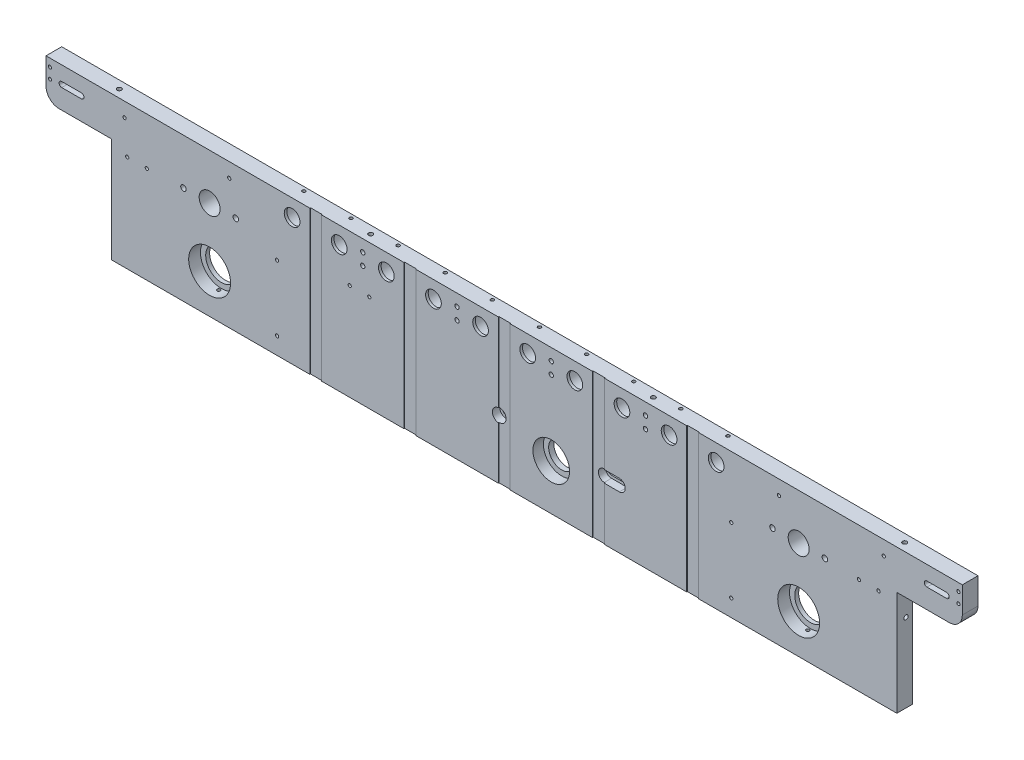
from build123d import *

# Parameters (mm, degrees)
EXTRUDE_1_DEPTH           = 12
FILLET_1_R                = 10
SKETCH_4_R                = 16
CUT_EXTRUDE_3_DEPTH       = 9
SKETCH_6_R                = 7.5
CUT_EXTRUDE_4_DEPTH       = 10
SKETCH_7_R                = 5.5
CUT_EXTRUDE_5_DEPTH       = 368.074924232
CUT_EXTRUDE_6_DEPTH       = 368.074924232
SKETCH_12_R               = 14
CUT_EXTRUDE_7_DEPTH       = 8
SKETCH_13_R               = 10
CUT_EXTRUDE_8_DEPTH       = 367.965938474
HOLE_WIZARD_M3_2_REACH    = 369.075
HOLE_WIZARD_M3_2_BORE_R   = 1.25
HOLE_WIZARD_M3_4_D        = 2.5
HOLE_WIZARD_2_D           = 5.5
HOLE_WIZARD_2_CBORE_D     = 10
HOLE_WIZARD_2_CBORE_DEPTH = 5.7
CUT_EXTRUDE_9_DEPTH       = 368.074924262
CUT_EXTRUDE_10_DEPTH      = 6
HOLE_WIZARD_M4_2_D        = 3.3
HOLE_WIZARD_M4_2_DEPTH    = 10
HOLE_WIZARD_M4_2_TIP      = 0.991420021
HOLE_WIZARD_M4_3_D        = 3.3
HOLE_WIZARD_M4_3_DEPTH    = 10.1
HOLE_WIZARD_M4_3_TIP      = 0.991420021
HOLE_WIZARD_M4_4_D        = 3.3
HOLE_WIZARD_M4_4_DEPTH    = 12.1
HOLE_WIZARD_M4_4_TIP      = 0.991420021
HOLE_WIZARD_M3_5_D        = 2.5
SKETCH_38_R               = 12
CUT_EXTRUDE_11_DEPTH      = 367.989100688
SKETCH_39_W               = 9
SKETCH_39_H               = 0.5
CUT_EXTRUDE_12_DEPTH      = 368.074924265
HOLE_WIZARD_M4_5_D        = 3.3
HOLE_WIZARD_M4_5_DEPTH    = 12
HOLE_WIZARD_M4_5_TIP      = 0.991420021
HOLE_WIZARD_M3_6_REACH    = 369.075
HOLE_WIZARD_M3_6_BORE_R   = 1.25
SKETCH_44_R               = 8
CUT_EXTRUDE_13_DEPTH      = 368.074924265
HOLE_WIZARD_M5_1_D        = 4.2
HOLE_WIZARD_3_D           = 2.4
HOLE_WIZARD_3_CBORE_D     = 4.3
HOLE_WIZARD_3_CBORE_DEPTH = 2.3
HOLE_WIZARD_4_D           = 2.4
HOLE_WIZARD_4_CBORE_D     = 4.3
HOLE_WIZARD_4_CBORE_DEPTH = 2.3
SKETCH_51_R               = 1.6
CUT_EXTRUDE_14_DEPTH      = 368.074924265
HOLE_WIZARD_M4_6_D        = 3.3
HOLE_WIZARD_5_D           = 12
HOLE_WIZARD_5_CBORE_D     = 16
HOLE_WIZARD_5_CBORE_DEPTH = 10
HOLE_WIZARD_M3_7_D        = 2.5


with BuildPart() as part:
    # 草图1 → 凸台-拉伸1 (new body)
    with BuildSketch(Plane.XY):
        Polygon((-350, -30), (-300, -30), (-300, -110), (300, -110), (300, -30), (350, -30), (350, 0), (-350, 0), align=None)
    extrude(amount=EXTRUDE_1_DEPTH)

    # 圆角1
    fillet_1_edges = [part.edges().sort_by_distance(p)[0] for p in [
        (350, -30, 6),
        (-350, -30, 6),
    ]]
    fillet(fillet_1_edges, radius=FILLET_1_R)

    # 草图4 → 切除-拉伸3 (cut)
    with BuildSketch(Plane.XY.offset(12)):
        with Locations((-225, -80)):
            Circle(SKETCH_4_R)
        with Locations(Location((225, -80, 0), (0, 0, 180))):
            Circle(SKETCH_4_R)
    extrude(amount=-CUT_EXTRUDE_3_DEPTH, mode=Mode.SUBTRACT)

    # 草图6 → 切除-拉伸4 (cut)
    with BuildSketch(Plane(origin=(0, 0, 0), x_dir=(-1, 0, 0), z_dir=(0, 0, -1))):
        with Locations((-162, -13)):
            Circle(SKETCH_6_R)
        with Locations((-126, -13)):
            Circle(SKETCH_6_R)
        with Locations((-90, -13)):
            Circle(SKETCH_6_R)
        with Locations((-54, -13)):
            Circle(SKETCH_6_R)
        with Locations((-18, -13)):
            Circle(SKETCH_6_R)
        with Locations((18, -13)):
            Circle(SKETCH_6_R)
        with Locations((54, -13)):
            Circle(SKETCH_6_R)
        with Locations((90, -13)):
            Circle(SKETCH_6_R)
        with Locations((126, -13)):
            Circle(SKETCH_6_R)
        with Locations((162, -13)):
            Circle(SKETCH_6_R)
    extrude(amount=-CUT_EXTRUDE_4_DEPTH, mode=Mode.SUBTRACT)

    # 草图7 → 切除-拉伸5 (cut, through all)
    with BuildSketch(Plane(origin=(0, 0, 0), x_dir=(-1, 0, 0), z_dir=(0, 0, -1))):
        with Locations((-162, -13)):
            Circle(SKETCH_7_R)
        with Locations((-126, -13)):
            Circle(SKETCH_7_R)
        with Locations((-90, -13)):
            Circle(SKETCH_7_R)
        with Locations((-54, -13)):
            Circle(SKETCH_7_R)
        with Locations((-18, -13)):
            Circle(SKETCH_7_R)
        with Locations((18, -13)):
            Circle(SKETCH_7_R)
        with Locations((54, -13)):
            Circle(SKETCH_7_R)
        with Locations((90, -13)):
            Circle(SKETCH_7_R)
        with Locations((126, -13)):
            Circle(SKETCH_7_R)
        with Locations((162, -13)):
            Circle(SKETCH_7_R)
    extrude(amount=-CUT_EXTRUDE_5_DEPTH, mode=Mode.SUBTRACT)

    # 草图8 → 切除-拉伸6 (cut, through all)
    with BuildSketch(Plane(origin=(0, 0, 0), x_dir=(-1, 0, 0), z_dir=(0, 0, -1))):
        with BuildLine():
            Line((-338, -11), (-323, -11))
            ThreePointArc((-323, -11), (-321, -13), (-323, -15))
            Line((-323, -15), (-338, -15))
            ThreePointArc((-338, -15), (-340, -13), (-338, -11))
        make_face()
        with BuildLine():
            Line((338, -11), (323, -11))
            ThreePointArc((323, -11), (321, -13), (323, -15))
            Line((323, -15), (338, -15))
            ThreePointArc((338, -15), (340, -13), (338, -11))
        make_face()
    extrude(amount=-CUT_EXTRUDE_6_DEPTH, mode=Mode.SUBTRACT)

    # 草图12 → 切除-拉伸7 (cut)
    with BuildSketch(Plane.XY.offset(12)):
        with Locations((36, -75)):
            Circle(SKETCH_12_R)
    extrude(amount=-CUT_EXTRUDE_7_DEPTH, mode=Mode.SUBTRACT)

    # 草图13 → 切除-拉伸8 (cut, through all)
    with BuildSketch(Plane.XY.offset(4)):
        with Locations((36, -75)):
            Circle(SKETCH_13_R)
    extrude(amount=-CUT_EXTRUDE_8_DEPTH, mode=Mode.SUBTRACT)

    # M3 螺纹孔2 bore → M3 螺纹孔2 (cut, up to next)
    with BuildSketch(Plane(origin=(0, -110, 0), x_dir=(-1, 0, 0), z_dir=(0, -1, 0)), mode=Mode.PRIVATE) as hole_wizard_m3_2_sk1:
        with Locations((225, -5)):
            Circle(HOLE_WIZARD_M3_2_BORE_R)
    hole_wizard_m3_2_tool1 = extrude(hole_wizard_m3_2_sk1.sketch, amount=-HOLE_WIZARD_M3_2_REACH, mode=Mode.PRIVATE) & part.part
    # M3 螺纹孔2 bore → M3 螺纹孔2 (cut, up to next)
    with BuildSketch(Plane(origin=(0, -110, 0), x_dir=(-1, 0, 0), z_dir=(0, -1, 0)), mode=Mode.PRIVATE) as hole_wizard_m3_2_sk2:
        with Locations((-225, -5)):
            Circle(HOLE_WIZARD_M3_2_BORE_R)
    hole_wizard_m3_2_tool2 = extrude(hole_wizard_m3_2_sk2.sketch, amount=-HOLE_WIZARD_M3_2_REACH, mode=Mode.PRIVATE) & part.part
    add(hole_wizard_m3_2_tool1.solids().sort_by_distance((-225, -110, 5))[0], mode=Mode.SUBTRACT)
    add(hole_wizard_m3_2_tool2.solids().sort_by_distance((225, -110, 5))[0], mode=Mode.SUBTRACT)

    # M3 螺纹孔4 (through all)
    with Locations(Plane.XY.offset(12)):
        with Locations((290, -11), (210, -11), (-210, -11), (-290, -11)):
            Hole(HOLE_WIZARD_M3_4_D / 2)

    # 打孔尺寸根据内六角圆柱头螺钉的类型2 (through all)
    with Locations(Plane.XY.offset(12)):
        with Locations((-4, -65)):
            CounterBoreHole(HOLE_WIZARD_2_D / 2, HOLE_WIZARD_2_CBORE_D / 2, HOLE_WIZARD_2_CBORE_DEPTH)

    # 草图28 → 切除-拉伸9 (cut, through all)
    with BuildSketch(Plane.XY.offset(12)):
        with BuildLine():
            Line((76, -62.5), (88, -62.5))
            ThreePointArc((88, -62.5), (90.5, -65), (88, -67.5))
            Line((88, -67.5), (76, -67.5))
            ThreePointArc((76, -67.5), (73.5, -65), (76, -62.5))
        make_face()
    extrude(amount=-CUT_EXTRUDE_9_DEPTH, mode=Mode.SUBTRACT)

    # 草图29 → 切除-拉伸10 (cut)
    with BuildSketch(Plane.XY.offset(12)):
        with BuildLine():
            Line((76, -60.5), (88, -60.5))
            ThreePointArc((88, -60.5), (92.5, -65), (88, -69.5))
            Line((88, -69.5), (76, -69.5))
            ThreePointArc((76, -69.5), (71.5, -65), (76, -60.5))
        make_face()
    extrude(amount=-CUT_EXTRUDE_10_DEPTH, mode=Mode.SUBTRACT)

    # M4 螺纹孔2
    with Locations(Plane(origin=(300, 0, 0), x_dir=(0, 0, -1), z_dir=(1, 0, 0))):
        with Locations((-5, -50)):
            Hole(HOLE_WIZARD_M4_2_D / 2, depth=HOLE_WIZARD_M4_2_DEPTH)
            with Locations((0, 0, -(HOLE_WIZARD_M4_2_DEPTH + HOLE_WIZARD_M4_2_TIP / 2))):  # 118° drill point
                Cone(0, HOLE_WIZARD_M4_2_D / 2, HOLE_WIZARD_M4_2_TIP, mode=Mode.SUBTRACT)

    # M4 螺纹孔3
    with Locations(Plane.ZY.offset(300)):
        with Locations((5, -50)):
            Hole(HOLE_WIZARD_M4_3_D / 2, depth=HOLE_WIZARD_M4_3_DEPTH)
            with Locations((0, 0, -(HOLE_WIZARD_M4_3_DEPTH + HOLE_WIZARD_M4_3_TIP / 2))):  # 118° drill point
                Cone(0, HOLE_WIZARD_M4_3_D / 2, HOLE_WIZARD_M4_3_TIP, mode=Mode.SUBTRACT)

    # M4 螺纹孔4
    with Locations(Plane(origin=(0, -110, 0), x_dir=(-1, 0, 0), z_dir=(0, -1, 0))):
        with Locations((262, -5), (82, -5), (-82, -5), (-262, -5)):
            Hole(HOLE_WIZARD_M4_4_D / 2, depth=HOLE_WIZARD_M4_4_DEPTH)
            with Locations((0, 0, -(HOLE_WIZARD_M4_4_DEPTH + HOLE_WIZARD_M4_4_TIP / 2))):  # 118° drill point
                Cone(0, HOLE_WIZARD_M4_4_D / 2, HOLE_WIZARD_M4_4_TIP, mode=Mode.SUBTRACT)

    # M3 螺纹孔5 (through all)
    with Locations(Plane.XY.offset(12)):
        with Locations((286, -36), (271, -36), (-118, -36), (-103, -36), (-273, -36), (-288, -36)):
            Hole(HOLE_WIZARD_M3_5_D / 2)

    # 草图38 → 切除-拉伸11 (cut, through all)
    with BuildSketch(Plane.XY.offset(3)):
        with Locations((225, -80)):
            Circle(SKETCH_38_R)
        with Locations((-225, -80)):
            Circle(SKETCH_38_R)
    extrude(amount=-CUT_EXTRUDE_11_DEPTH, mode=Mode.SUBTRACT)

    # 草图39 → 切除-拉伸12 (cut, through all)
    with BuildSketch(Plane(origin=(0, 0, 0), x_dir=(1, 0, 0), z_dir=(0, 1, 0))):
        with Locations((-144, -11.75)):
            Rectangle(SKETCH_39_W, SKETCH_39_H)
        with Locations((-72, -11.75)):
            Rectangle(SKETCH_39_W, SKETCH_39_H)
        with Locations((0, -11.75)):
            Rectangle(SKETCH_39_W, SKETCH_39_H)
        with Locations((72, -11.75)):
            Rectangle(SKETCH_39_W, SKETCH_39_H)
        with Locations((144, -11.75)):
            Rectangle(SKETCH_39_W, SKETCH_39_H)
    extrude(amount=-CUT_EXTRUDE_12_DEPTH, mode=Mode.SUBTRACT)

    # M4 螺纹孔5
    with Locations(Plane(origin=(0, 0, 0), x_dir=(1, 0, 0), z_dir=(0, 1, 0))):
        with Locations((-300.000000001, -6), (-108.000000001, -6), (107.999999999, -6), (299.999999999, -6)):
            Hole(HOLE_WIZARD_M4_5_D / 2, depth=HOLE_WIZARD_M4_5_DEPTH)
            with Locations((0, 0, -(HOLE_WIZARD_M4_5_DEPTH + HOLE_WIZARD_M4_5_TIP / 2))):  # 118° drill point
                Cone(0, HOLE_WIZARD_M4_5_D / 2, HOLE_WIZARD_M4_5_TIP, mode=Mode.SUBTRACT)

    # M3 螺纹孔6 bore → M3 螺纹孔6 (cut, up to next)
    with BuildSketch(Plane(origin=(0, 0, 0), x_dir=(1, 0, 0), z_dir=(0, 1, 0)), mode=Mode.PRIVATE) as hole_wizard_m3_6_sk1:
        with Locations((-162, -3)):
            Circle(HOLE_WIZARD_M3_6_BORE_R)
    hole_wizard_m3_6_tool1 = extrude(hole_wizard_m3_6_sk1.sketch, amount=-HOLE_WIZARD_M3_6_REACH, mode=Mode.PRIVATE) & part.part
    # M3 螺纹孔6 bore → M3 螺纹孔6 (cut, up to next)
    with BuildSketch(Plane(origin=(0, 0, 0), x_dir=(1, 0, 0), z_dir=(0, 1, 0)), mode=Mode.PRIVATE) as hole_wizard_m3_6_sk2:
        with Locations((-126, -3)):
            Circle(HOLE_WIZARD_M3_6_BORE_R)
    hole_wizard_m3_6_tool2 = extrude(hole_wizard_m3_6_sk2.sketch, amount=-HOLE_WIZARD_M3_6_REACH, mode=Mode.PRIVATE) & part.part
    # M3 螺纹孔6 bore → M3 螺纹孔6 (cut, up to next)
    with BuildSketch(Plane(origin=(0, 0, 0), x_dir=(1, 0, 0), z_dir=(0, 1, 0)), mode=Mode.PRIVATE) as hole_wizard_m3_6_sk3:
        with Locations((-90, -3)):
            Circle(HOLE_WIZARD_M3_6_BORE_R)
    hole_wizard_m3_6_tool3 = extrude(hole_wizard_m3_6_sk3.sketch, amount=-HOLE_WIZARD_M3_6_REACH, mode=Mode.PRIVATE) & part.part
    # M3 螺纹孔6 bore → M3 螺纹孔6 (cut, up to next)
    with BuildSketch(Plane(origin=(0, 0, 0), x_dir=(1, 0, 0), z_dir=(0, 1, 0)), mode=Mode.PRIVATE) as hole_wizard_m3_6_sk4:
        with Locations((-54, -3)):
            Circle(HOLE_WIZARD_M3_6_BORE_R)
    hole_wizard_m3_6_tool4 = extrude(hole_wizard_m3_6_sk4.sketch, amount=-HOLE_WIZARD_M3_6_REACH, mode=Mode.PRIVATE) & part.part
    # M3 螺纹孔6 bore → M3 螺纹孔6 (cut, up to next)
    with BuildSketch(Plane(origin=(0, 0, 0), x_dir=(1, 0, 0), z_dir=(0, 1, 0)), mode=Mode.PRIVATE) as hole_wizard_m3_6_sk5:
        with Locations((-18, -3)):
            Circle(HOLE_WIZARD_M3_6_BORE_R)
    hole_wizard_m3_6_tool5 = extrude(hole_wizard_m3_6_sk5.sketch, amount=-HOLE_WIZARD_M3_6_REACH, mode=Mode.PRIVATE) & part.part
    # M3 螺纹孔6 bore → M3 螺纹孔6 (cut, up to next)
    with BuildSketch(Plane(origin=(0, 0, 0), x_dir=(1, 0, 0), z_dir=(0, 1, 0)), mode=Mode.PRIVATE) as hole_wizard_m3_6_sk6:
        with Locations((18, -3)):
            Circle(HOLE_WIZARD_M3_6_BORE_R)
    hole_wizard_m3_6_tool6 = extrude(hole_wizard_m3_6_sk6.sketch, amount=-HOLE_WIZARD_M3_6_REACH, mode=Mode.PRIVATE) & part.part
    # M3 螺纹孔6 bore → M3 螺纹孔6 (cut, up to next)
    with BuildSketch(Plane(origin=(0, 0, 0), x_dir=(1, 0, 0), z_dir=(0, 1, 0)), mode=Mode.PRIVATE) as hole_wizard_m3_6_sk7:
        with Locations((54, -3)):
            Circle(HOLE_WIZARD_M3_6_BORE_R)
    hole_wizard_m3_6_tool7 = extrude(hole_wizard_m3_6_sk7.sketch, amount=-HOLE_WIZARD_M3_6_REACH, mode=Mode.PRIVATE) & part.part
    # M3 螺纹孔6 bore → M3 螺纹孔6 (cut, up to next)
    with BuildSketch(Plane(origin=(0, 0, 0), x_dir=(1, 0, 0), z_dir=(0, 1, 0)), mode=Mode.PRIVATE) as hole_wizard_m3_6_sk8:
        with Locations((90, -3)):
            Circle(HOLE_WIZARD_M3_6_BORE_R)
    hole_wizard_m3_6_tool8 = extrude(hole_wizard_m3_6_sk8.sketch, amount=-HOLE_WIZARD_M3_6_REACH, mode=Mode.PRIVATE) & part.part
    # M3 螺纹孔6 bore → M3 螺纹孔6 (cut, up to next)
    with BuildSketch(Plane(origin=(0, 0, 0), x_dir=(1, 0, 0), z_dir=(0, 1, 0)), mode=Mode.PRIVATE) as hole_wizard_m3_6_sk9:
        with Locations((126, -3)):
            Circle(HOLE_WIZARD_M3_6_BORE_R)
    hole_wizard_m3_6_tool9 = extrude(hole_wizard_m3_6_sk9.sketch, amount=-HOLE_WIZARD_M3_6_REACH, mode=Mode.PRIVATE) & part.part
    # M3 螺纹孔6 bore → M3 螺纹孔6 (cut, up to next)
    with BuildSketch(Plane(origin=(0, 0, 0), x_dir=(1, 0, 0), z_dir=(0, 1, 0)), mode=Mode.PRIVATE) as hole_wizard_m3_6_sk10:
        with Locations((162, -3)):
            Circle(HOLE_WIZARD_M3_6_BORE_R)
    hole_wizard_m3_6_tool10 = extrude(hole_wizard_m3_6_sk10.sketch, amount=-HOLE_WIZARD_M3_6_REACH, mode=Mode.PRIVATE) & part.part
    add(hole_wizard_m3_6_tool1.solids().sort_by_distance((-162, 0, 3))[0], mode=Mode.SUBTRACT)
    add(hole_wizard_m3_6_tool2.solids().sort_by_distance((-126, 0, 3))[0], mode=Mode.SUBTRACT)
    add(hole_wizard_m3_6_tool3.solids().sort_by_distance((-90, 0, 3))[0], mode=Mode.SUBTRACT)
    add(hole_wizard_m3_6_tool4.solids().sort_by_distance((-54, 0, 3))[0], mode=Mode.SUBTRACT)
    add(hole_wizard_m3_6_tool5.solids().sort_by_distance((-18, 0, 3))[0], mode=Mode.SUBTRACT)
    add(hole_wizard_m3_6_tool6.solids().sort_by_distance((18, 0, 3))[0], mode=Mode.SUBTRACT)
    add(hole_wizard_m3_6_tool7.solids().sort_by_distance((54, 0, 3))[0], mode=Mode.SUBTRACT)
    add(hole_wizard_m3_6_tool8.solids().sort_by_distance((90, 0, 3))[0], mode=Mode.SUBTRACT)
    add(hole_wizard_m3_6_tool9.solids().sort_by_distance((126, 0, 3))[0], mode=Mode.SUBTRACT)
    add(hole_wizard_m3_6_tool10.solids().sort_by_distance((162, 0, 3))[0], mode=Mode.SUBTRACT)

    # 草图44 → 切除-拉伸13 (cut, through all)
    with BuildSketch(Plane.XY.offset(12)):
        with Locations((-225, -35)):
            Circle(SKETCH_44_R)
        with Locations((225, -35)):
            Circle(SKETCH_44_R)
    extrude(amount=-CUT_EXTRUDE_13_DEPTH, mode=Mode.SUBTRACT)

    # M5 螺纹孔1 (through all)
    with Locations(Plane.XY.offset(12)):
        with Locations((245, -35), (205, -35), (-205, -35), (-245, -35)):
            Hole(HOLE_WIZARD_M5_1_D / 2)

    # 打孔尺寸根据内六角圆柱头螺钉的类型3 (through all)
    with Locations(Plane(origin=(0, 0, 0), x_dir=(-1, 0, 0), z_dir=(0, 0, -1))):
        with Locations((-347, -6), (-347, -14)):
            CounterBoreHole(HOLE_WIZARD_3_D / 2, HOLE_WIZARD_3_CBORE_D / 2, HOLE_WIZARD_3_CBORE_DEPTH)

    # 打孔尺寸根据内六角圆柱头螺钉的类型4 (through all)
    with Locations(Plane(origin=(0, 0, 0), x_dir=(-1, 0, 0), z_dir=(0, 0, -1))):
        with Locations((347, -6), (347, -14)):
            CounterBoreHole(HOLE_WIZARD_4_D / 2, HOLE_WIZARD_4_CBORE_D / 2, HOLE_WIZARD_4_CBORE_DEPTH)

    # 草图51 → 切除-拉伸14 (cut, through all)
    with BuildSketch(Plane.XY.offset(12)):
        with Locations((108, -9)):
            Circle(SKETCH_51_R)
        with Locations((108, -18)):
            Circle(SKETCH_51_R)
        with Locations((36, -18)):
            Circle(SKETCH_51_R)
        with Locations((36, -9)):
            Circle(SKETCH_51_R)
        with Locations((-36, -18)):
            Circle(SKETCH_51_R)
        with Locations((-36, -9)):
            Circle(SKETCH_51_R)
        with Locations((-108, -18)):
            Circle(SKETCH_51_R)
        with Locations((-108, -9)):
            Circle(SKETCH_51_R)
    extrude(amount=-CUT_EXTRUDE_14_DEPTH, mode=Mode.SUBTRACT)

    # M4 螺纹孔6 (through all)
    with Locations(Plane(origin=(0, 0, 0), x_dir=(-1, 0, 0), z_dir=(0, 0, -1))):
        with Locations((-108, -9), (-108, -18), (-36, -9), (-36, -18), (36, -9), (36, -18), (108, -9), (108, -18)):
            Hole(HOLE_WIZARD_M4_6_D / 2)

    # 打孔尺寸根据内六角圆柱头螺钉的类型5 (through all)
    with Locations(Plane(origin=(0, 0, 0), x_dir=(-1, 0, 0), z_dir=(0, 0, -1))):
        with Locations((-162, -13), (-126, -13), (-90, -13), (-54, -13), (-18, -13), (18, -13), (54, -13), (90, -13), (126, -13), (162, -13)):
            CounterBoreHole(HOLE_WIZARD_5_D / 2, HOLE_WIZARD_5_CBORE_D / 2, HOLE_WIZARD_5_CBORE_DEPTH)

    # M3 螺纹孔7 (through all)
    with Locations(Plane(origin=(0, 0, 0), x_dir=(-1, 0, 0), z_dir=(0, 0, -1))):
        with Locations((173.5, -97), (173.5, -47), (-173.5, -97), (-173.5, -47)):
            Hole(HOLE_WIZARD_M3_7_D / 2)


solid = part.part
